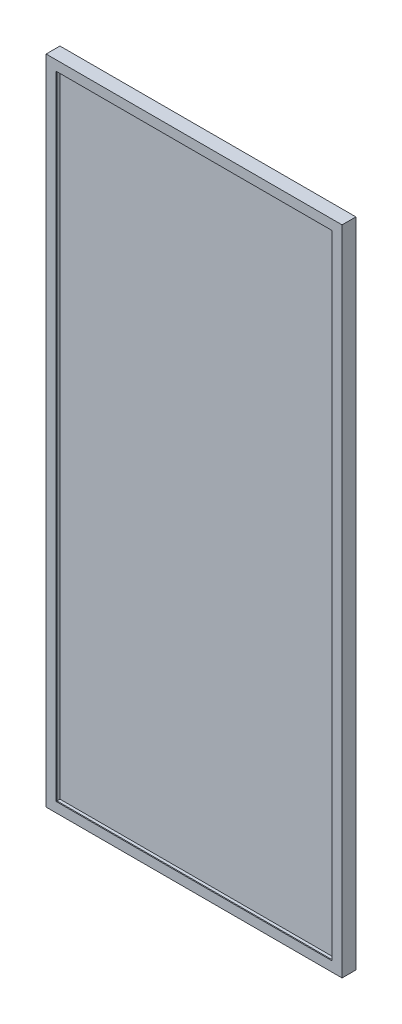
SolidWorks part; units mm, degrees
ref_plane "前视基准面" through (0, 0, 0) normal (0, 0, 1) x (1, 0, 0)
ref_plane "上视基准面" through (0, 0, 0) normal (0, 1, 0) x (1, 0, 0)
ref_plane "右视基准面" through (0, 0, 0) normal (1, 0, 0) x (0, 0, -1)
sketch "草图1" plane through (0, 0, 0) normal (0, 0, 1) x (1, 0, 0)
  line L1 (0, 0) -> (598.5, 0)
  line L2 (0, 0) -> (0, 1319)
  line L3 (0, 1319) -> (598.5, 1319)
  line L4 (598.5, 0) -> (598.5, 1319)
  dimension "D1" = 1319
  dimension "D2" = 598.5
extrude "凸台-拉伸1" add sketch "草图1" along normal blind 28
shell "抽壳1" thickness 2
sketch "草图2" plane through (0, 0, 28) normal (0, 0, 1) x (1, 0, 0)
  line L14 (20, 1299) -> (20, 20)
  line L15 (20, 20) -> (578.5, 20)
  line L16 (578.5, 20) -> (578.5, 1299)
  line L17 (578.5, 1299) -> (20, 1299)
  line L18 (20, 1299) -> (20, 20)
  line L19 (20, 20) -> (578.5, 20)
  line L20 (578.5, 20) -> (578.5, 1299)
  line L21 (578.5, 1299) -> (20, 1299)
  line L26 (0, 1319) -> (0, 0)
  line L27 (0, 0) -> (598.5, 0)
  line L28 (598.5, 0) -> (598.5, 1319)
  line L29 (598.5, 1319) -> (0, 1319)
  line L30 (0, 1319) -> (0, 0)
  line L31 (0, 0) -> (598.5, 0)
  line L32 (598.5, 0) -> (598.5, 1319)
  line L33 (598.5, 1319) -> (0, 1319)
  dimension "D1" = 20
  dimension "D2" = 0
extrude "凸台-拉伸2" add sketch "草图2" against normal blind 2
